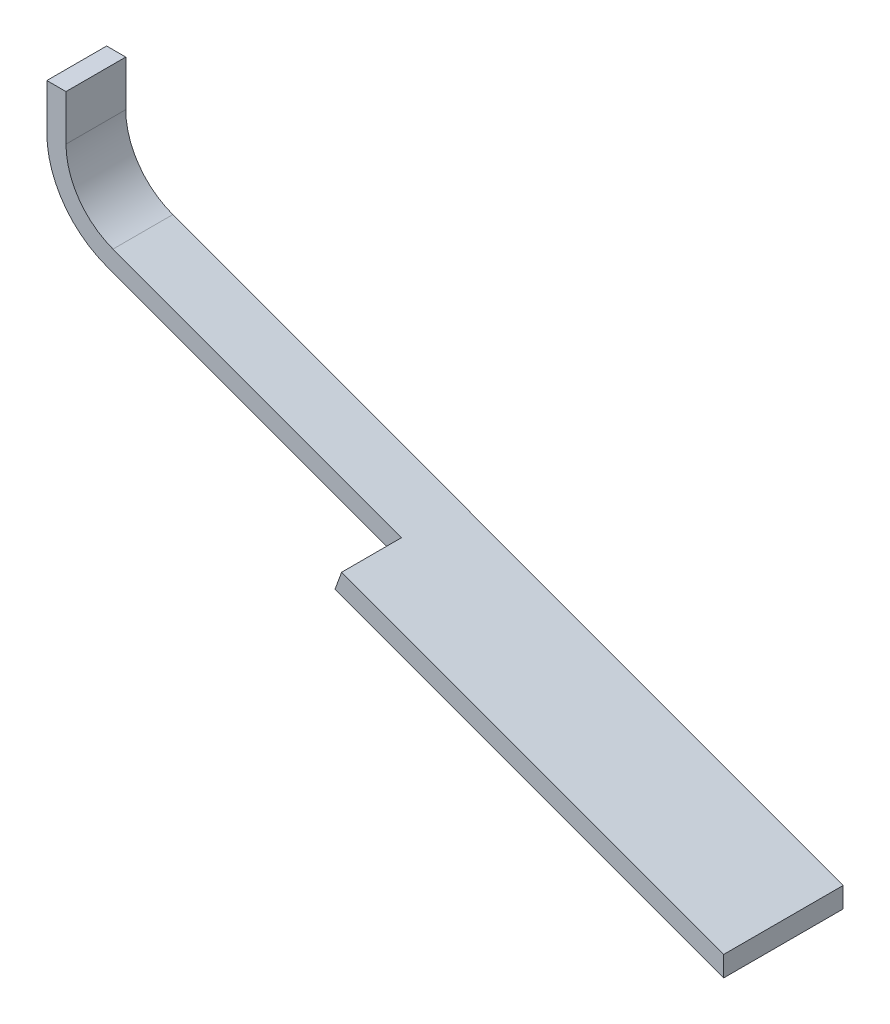
SolidWorks part; units mm, degrees
ref_plane "前视基准面" through (0, 0, 0) normal (0, 0, 1) x (1, 0, 0)
ref_plane "上视基准面" through (0, 0, 0) normal (0, 1, 0) x (1, 0, 0)
ref_plane "右视基准面" through (0, 0, 0) normal (1, 0, 0) x (0, 0, -1)
sketch "草图1" plane through (0, 0, 0) normal (0, 0, 1) x (1, 0, 0)
  line L0 (-158.4998, 75.4998) -> (-158.4998, 56.4529)
  line L1 (-133.5815, 20.7756) -> (146.7461, -82.0112)
  line L2 (-150.4998, 75.4998) -> (-150.4998, 56.4529)
  line L3 (-130.8275, 28.2866) -> (149.5002, -74.5002)
  line L4 (-158.4998, 75.4998) -> (-150.4998, 75.4998)
  line L5 (149.5002, -74.5002) -> (149.5002, -83.021)
  line L6 (146.7461, -82.0112) -> (149.5002, -83.021)
  arc A0 (-150.4998, 56.4529) -> (-130.8275, 28.2866) centre (-120.4998, 56.4529) ccw
  arc A1 (-158.4998, 56.4529) -> (-133.5815, 20.7756) centre (-120.4998, 56.4529) ccw
  dimension "D1" = 30
  dimension "D2" = 8
extrude "凸台-拉伸1" add sketch "草图1" along normal blind 50
sketch "草图2" plane through (-9.116, -24.8617, 0) normal (-0.3443, -0.9389, 0) x (0.9389, -0.3443, 0)
  line L0 (168.9425, 50) -> (-177.1686, 50)
  line L1 (-4.113, 50) -> (-4.113, 25)
  line L2 (-4.113, 25) -> (-4.113, 0)
  line L3 (-132.5686, 0) -> (168.9425, 0) construction
  line L4 (-4.113, 25) -> (-174.8029, 25)
  line L5 (-174.8029, 50) -> (-174.8029, 0) construction
  line L6 (-174.8029, 25) -> (-174.8029, 0)
  line L7 (-174.8029, 0) -> (-4.113, 0)
  line L8 (-174.8029, 25) -> (-174.8029, 50)
  line M4 (-132.5686, 50) -> (-132.5686, 0)
extrude "切除-拉伸1" cut sketch "草图2" against normal blind 49 contours L4 L1 L0 M4 | L8 L4 L0 M4
